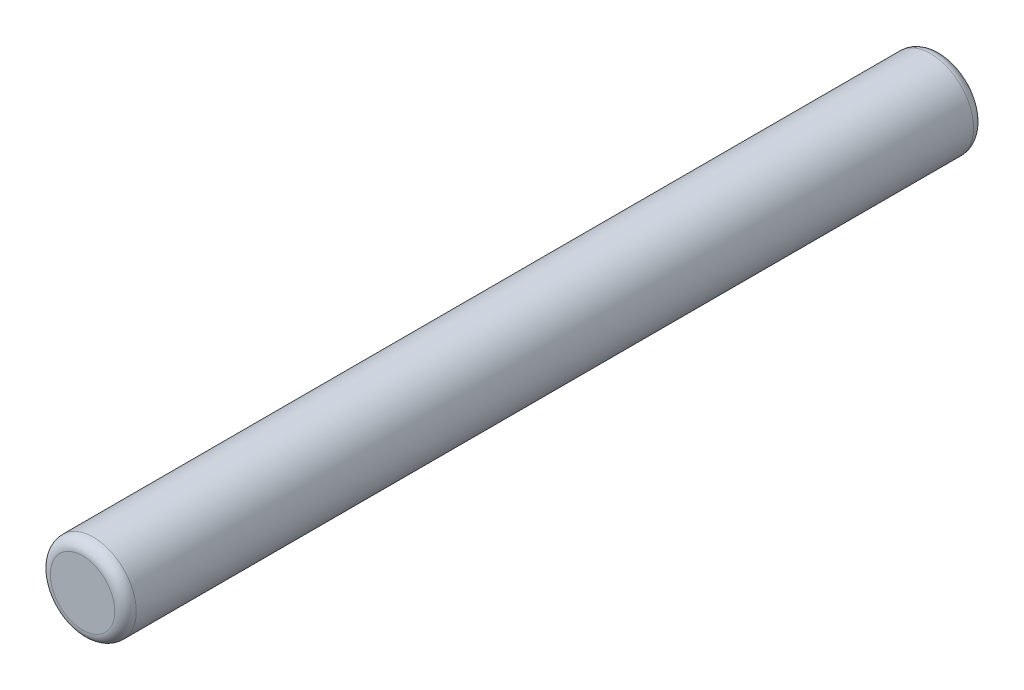
from build123d import *

# Parameters (mm, degrees)
BOSS_EXTRUDE1_DEPTH      = 20
BOSS_EXTRUDE1_DEPTH_BACK = 380
SKETCH1_R                = 20
FILLET1_R                = 5


with BuildPart() as part:
    # Sketch1 → Boss-Extrude1 (new, two sides: drawn at the far end of the back side and taken through both)
    with BuildSketch(Plane.XY.offset(-BOSS_EXTRUDE1_DEPTH_BACK)):
        with Locations((-290, 235)):
            Circle(SKETCH1_R)
    extrude(amount=BOSS_EXTRUDE1_DEPTH + BOSS_EXTRUDE1_DEPTH_BACK)

    # Fillet1
    fillet1_edges = [part.edges().sort_by_distance(p)[0] for p in [
        (-310, 235, 20),
        (-310, 235, -380),
    ]]
    fillet(fillet1_edges, radius=FILLET1_R)


solid = part.part
